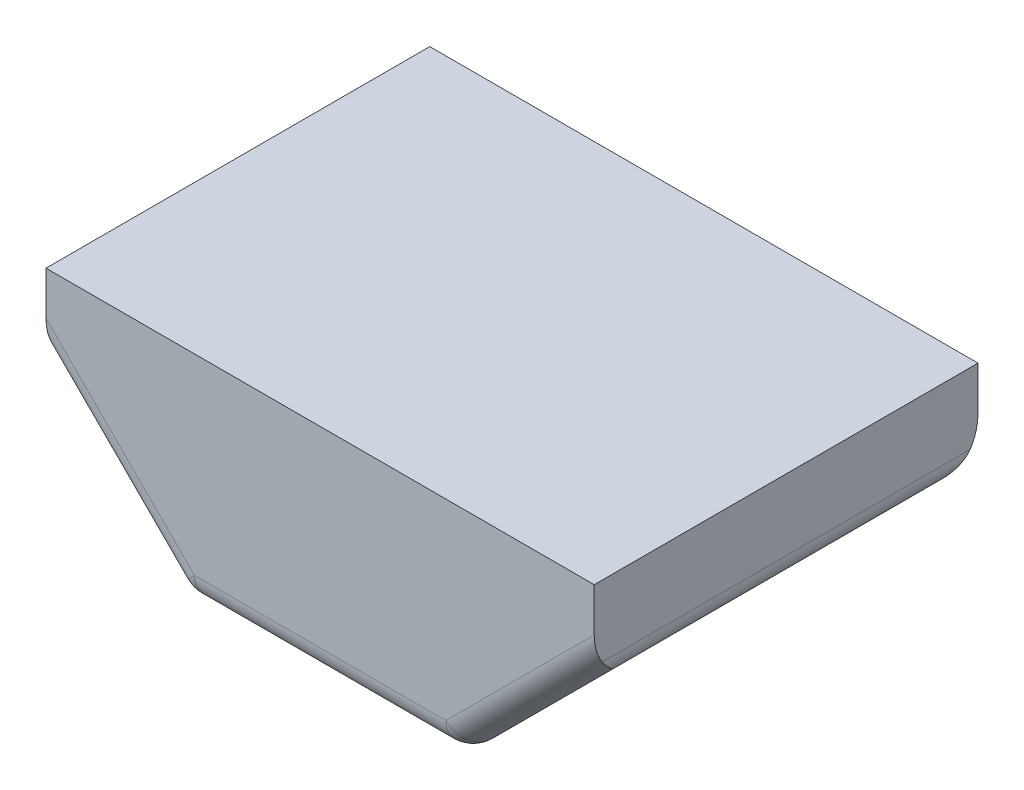
SolidWorks part; units mm, degrees
material "橡胶"
ref_plane "前视基准面" through (0, 0, 0) normal (0, 0, 1) x (1, 0, 0)
ref_plane "上视基准面" through (0, 0, 0) normal (0, 1, 0) x (1, 0, 0)
ref_plane "右视基准面" through (0, 0, 0) normal (1, 0, 0) x (0, 0, -1)
sketch "草图1" plane through (0, 0, 0) normal (0, 0, 1) x (1, 0, 0)
  line L0 (0, 0) -> (100, 0)
  line L1 (100, 0) -> (100, -15)
  line L2 (0, 0) -> (0, -15)
  line L5 (50, -40) -> (75, -40)
  line L6 (50, -40) -> (25, -40)
  line L7 (25, -40) -> (0, -15)
  line L8 (75, -40) -> (100, -15)
extrude "凸台-拉伸1" add sketch "草图1" along normal blind 70
fillet "圆角1" radius 5 10 edges at (75, -40, 35) (87.5, -27.5, 70) (100, -15, 35) (87.5, -27.5, 0) (0, -15, 35) (12.5, -27.5, 70) (25, -40, 35) (12.5, -27.5, 0) (50, -40, 0) (50, -40, 70)
